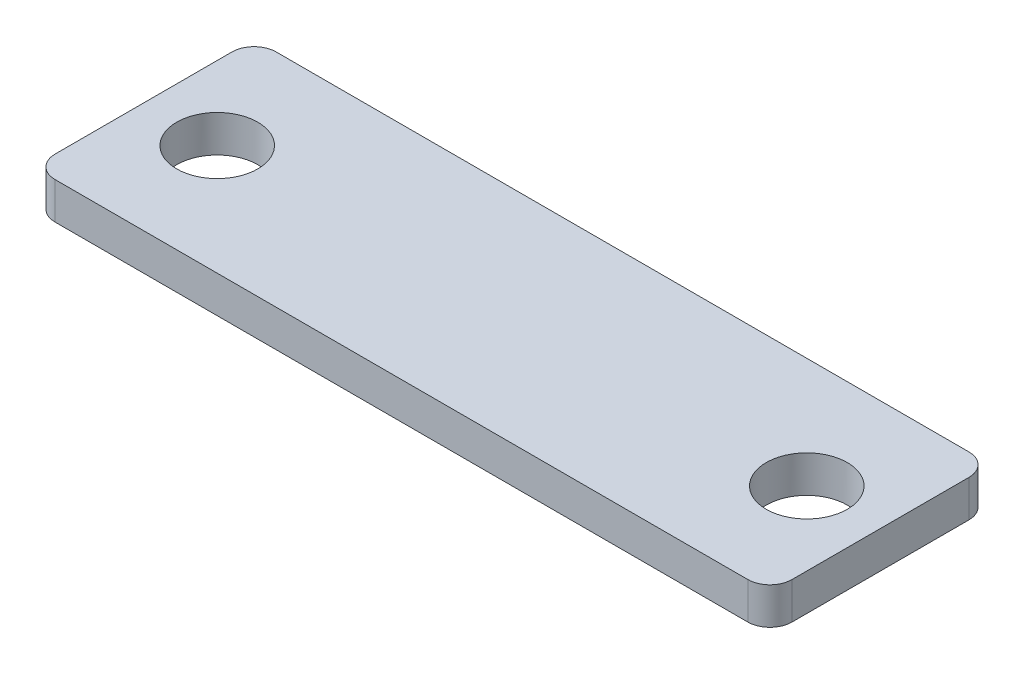
from build123d import *

# Parameters (mm, degrees)
SKETCH1_W           = 100
SKETCH1_H           = 30
BOSS_EXTRUDE1_DEPTH = 5
FILLET1_R           = 3
SKETCH3_R           = 5.5
CUT_EXTRUDE1_DEPTH  = 10


with BuildPart() as part:
    # Sketch1 → Boss-Extrude1 (new body)
    with BuildSketch(Plane(origin=(0, 0, 0), x_dir=(1, 0, 0), z_dir=(0, 1, 0))):
        Rectangle(SKETCH1_W, SKETCH1_H)
    extrude(amount=BOSS_EXTRUDE1_DEPTH)

    # Fillet1
    fillet1_edges = [part.edges().sort_by_distance(p)[0] for p in [
        (50, 2.5, 15),
        (-50, 2.5, 15),
        (-50, 2.5, -15),
        (50, 2.5, -15),
    ]]
    fillet(fillet1_edges, radius=FILLET1_R)

    # Sketch3 → Cut-Extrude1 (cut)
    with BuildSketch(Plane(origin=(0, 5, 0), x_dir=(1, 0, 0), z_dir=(0, 1, 0))):
        with Locations(Location((-40, 0, 0), (0, 0, 270))):
            Circle(SKETCH3_R)
        with Locations(Location((40, 0, 0), (0, 0, 270))):
            Circle(SKETCH3_R)
    extrude(amount=-CUT_EXTRUDE1_DEPTH, mode=Mode.SUBTRACT)


solid = part.part
